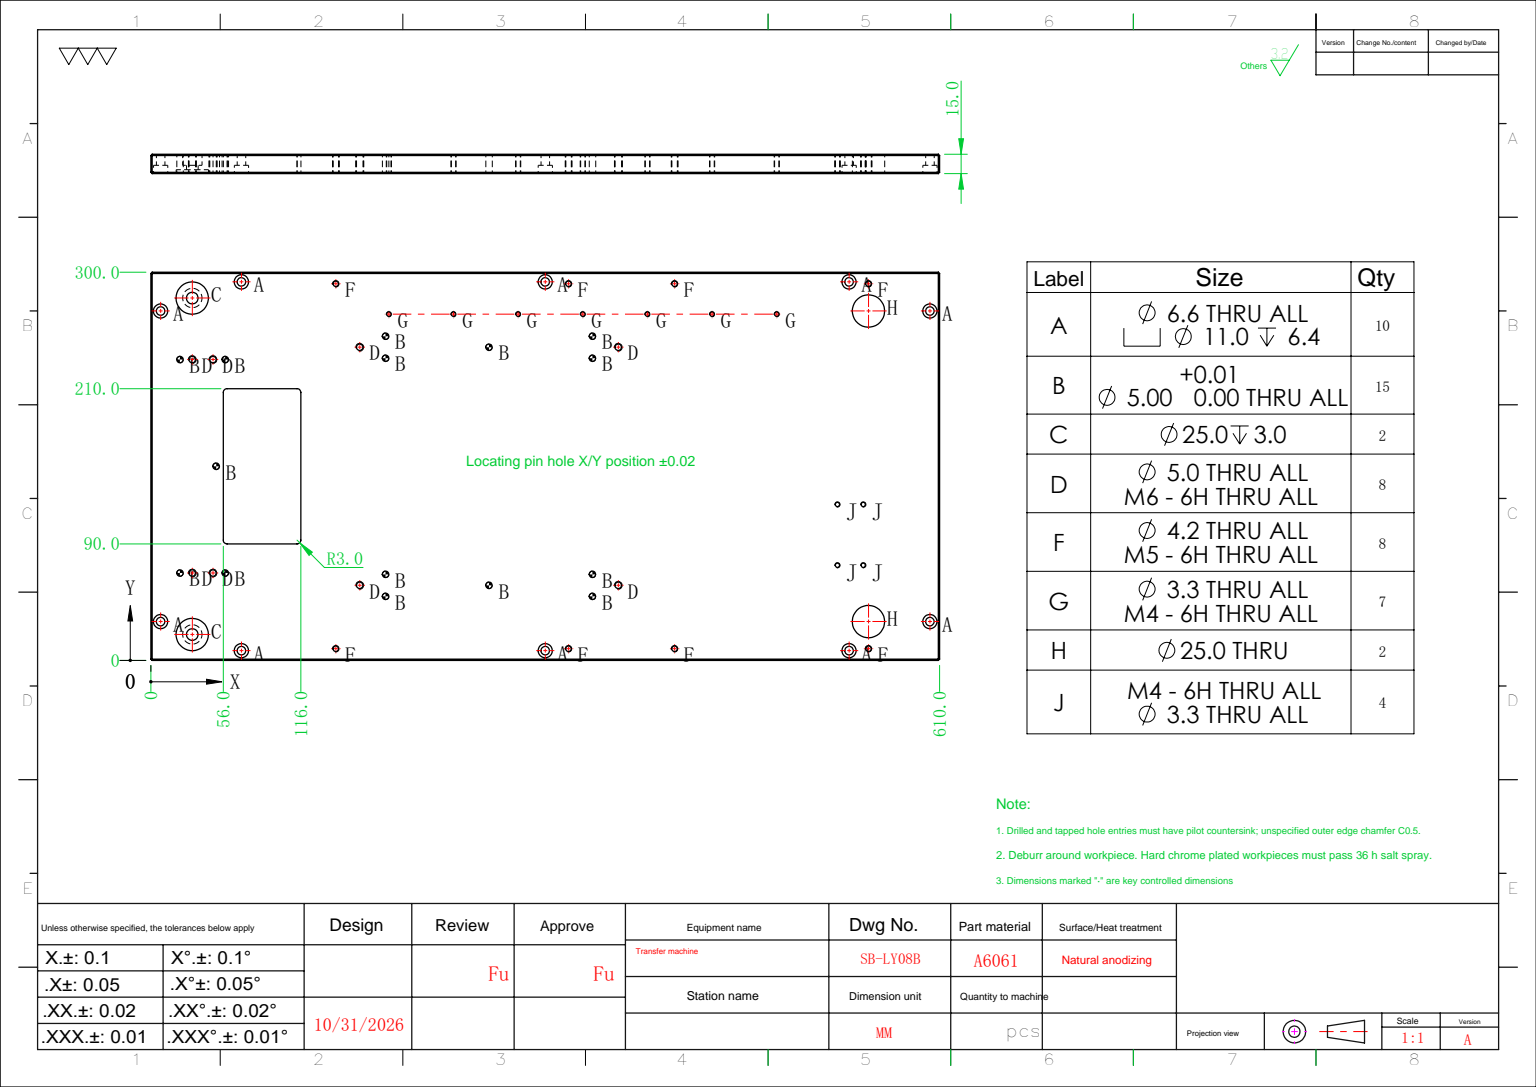
SolidWorks part; units mm, degrees
ref_plane "前视基准面" through (0, 0, 0) normal (0, 0, 1) x (1, 0, 0)
ref_plane "上视基准面" through (0, 0, 0) normal (0, 1, 0) x (1, 0, 0)
ref_plane "右视基准面" through (0, 0, 0) normal (1, 0, 0) x (0, 0, -1)
sketch "草图1" plane through (0, 0, 0) normal (0, 0, 1) x (1, 0, 0)
  line L1 (-305, -150) -> (305, -150)
  line L2 (-305, -150) -> (-305, 150)
  line L3 (-305, 150) -> (305, 150)
  line L4 (305, -150) -> (305, 150)
  line L5 (-305, -150) -> (305, 150) construction
  line L6 (-305, 150) -> (305, -150) construction
  point P0 (0, 0)
  dimension "D1" = 610
  dimension "D2" = 300
extrude "凸台-拉伸1" add sketch "草图1" along normal blind 15
sketch "草图25" plane through (0, 0, 15) normal (0, 0, 1) x (1, 0, 0)
  line L0 (0, 0) -> (254.8219, 0) construction
  line L1 (305, -150) -> (305, 150) construction
  circle A0 centre (273, -130) radius 12.5
  circle A1 centre (273, 130) radius 12.5
  dimension "D1" = 25
  dimension "D2" = 260
  dimension "D3" = 32
extrude "切除-拉伸4" cut sketch "草图25" against normal blind 3
sketch "草图26" plane through (0, 0, 15) normal (0, 0, 1) x (1, 0, 0)
  line L0 (0, 0) -> (330.7234, 0) construction
  line L1 (189, -60) -> (249, -60)
  line L2 (189, -60) -> (189, 60)
  line L3 (189, 60) -> (249, 60)
  line L4 (249, -60) -> (249, 60)
  line L5 (305, -150) -> (305, 150) construction
  dimension "D1" = 120
  dimension "D2" = 56
  dimension "D3" = 60
extrude "切除-拉伸5" cut sketch "草图26" against normal through all
hole_wizard "M6 螺纹孔1" positions "草图27" profile "草图28" tap size "M6" standard "ISO" end condition through all
sketch "草图27" plane through (0, 0, 15) normal (0, 0, 1) x (1, 0, 0)
  line L0 (0, 0) -> (315.5275, 0) construction
  line L2 (305, -150) -> (305, 150) construction
  point P0 (143.5008, -92)
  point P3 (-56.4992, -92)
  point P12 (-56.4992, 92)
  point P13 (143.5008, 92)
  dimension "D1" = 184
  dimension "D2" = 161.4992
  dimension "D3" = 200
sketch "草图28" plane through (143.5008, -92, 15) normal (1, 0, 0) x (0, -1, 0)
  line L0 (0, 0) -> (0, 15)
  line L1 (0, 15) -> (2.5, 15)
  line L2 (2.5, 15) -> (2.5, 0)
  line L5 (2.5, 0) -> (0, 0)
  line L11 (0, -6.35) -> (0, 107.95) construction
  dimension "通孔螺纹孔钻头直径" = 5
  dimension "通孔螺纹孔钻头深度" = 15
cosmetic thread "孔螺蚊线1" parameters "D2"=6
cosmetic thread "孔螺蚊线2" parameters "D2"=6
cosmetic thread "孔螺蚊线3" parameters "D2"=6
cosmetic thread "孔螺蚊线4" parameters "D2"=6
hole_wizard "大小mm 暗销孔1" positions "草图29" profile "草图30" hole size "Ø5.0" standard "ISO" end condition through all
sketch "草图29" plane through (0, 0, 15) normal (0, 0, 1) x (1, 0, 0)
  line L0 (-56.4992, -92) -> (143.5008, -92) construction
  line L3 (43.5008, -92) -> (43.5008, -134.7287) construction
  line L5 (0, 0) -> (308.2211, 0) construction
  circle A0 centre (143.5008, -92) radius 2.5 construction
  point P0 (123.5008, -83.5)
  point P2 (123.5008, -100.5)
  point P14 (43.5008, -92)
  point P18 (-36.4992, -100.5)
  point P19 (-36.4992, -83.5)
  point P25 (-36.4992, 83.5)
  point P26 (-36.4992, 100.5)
  point P27 (123.5008, 100.5)
  point P28 (123.5008, 83.5)
  point P32 (43.5008, 92)
  dimension "D1" = 17
  dimension "D2" = 20
sketch "草图30" plane through (123.5008, -83.5, 15) normal (1, 0, 0) x (0, -1, 0)
  line L0 (0, 0) -> (0, 15)
  line L1 (0, 15) -> (2.5, 15)
  line L2 (2.5, 15) -> (2.5, 0)
  line L5 (2.5, 0) -> (0, 0)
  line L11 (0, -6.35) -> (0, 107.95) construction
  dimension "通孔孔直径" = 5
  dimension "通孔孔深度" = 15
hole_wizard "M8 六角凹头螺钉的柱形沉头孔1" positions "草图31" profile "草图32" counterbore size "M8" standard "ISO" end condition through all
sketch "草图31" plane through (0, 0, 0) normal (0, 0, -1) x (-1, 0, 0)
  point P0 (-273, -130)
  point P3 (-273, 130)
sketch "草图32" plane through (273, -130, 0) normal (1, 0, 0) x (0, 1, 0)
  line L0 (0, 0) -> (0, 15)
  line L1 (0, 15) -> (4.5, 15)
  line L3 (4.5, 15) -> (4.5, 8.6)
  line L4 (4.5, 8.6) -> (7.5, 8.6)
  line L5 (7.5, 8.6) -> (7.5, 0)
  line L7 (7.5, 0) -> (0, 0)
  line L11 (0, -6.35) -> (0, 107.95) construction
  dimension "通孔孔直径" = 9
  dimension "通孔孔深度" = 15
  dimension "柱形沉头孔直径" = 15
  dimension "柱形沉头孔深度" = 8.6
hole_wizard "大小mm 暗销孔0" positions "草图33" profile "草图34" hole size "Ø5.0" standard "ISO" end condition through all
sketch "草图33" plane through (0, 0, 15) normal (0, 0, 1) x (1, 0, 0)
  line L0 (305, 0) -> (216.232, 0) construction
  line L1 (305, -150) -> (305, 150) construction
  line L2 (265, -90) -> (265, 90) construction
  point P0 (282.5, -82.5)
  point P2 (282.5, 82.5)
  point P33 (247.5, 82.5)
  point P34 (247.5, -82.5)
  point P35 (254.5, 0)
  dimension "D1" = 165
  dimension "D2" = 22.5
  dimension "D3" = 40
  dimension "D4" = 28
sketch "草图34" plane through (282.5, -82.5, 15) normal (1, 0, 0) x (0, -1, 0)
  line L0 (0, 0) -> (0, 15)
  line L1 (0, 15) -> (2.5, 15)
  line L2 (2.5, 15) -> (2.5, 0)
  line L5 (2.5, 0) -> (0, 0)
  line L11 (0, -6.35) -> (0, 107.95) construction
  dimension "通孔孔直径" = 5
  dimension "通孔孔深度" = 15
hole_wizard "M6 螺纹孔2" positions "草图35" profile "草图36" tap size "M6" standard "ISO" end condition through all
sketch "草图35" plane through (0, 0, 15) normal (0, 0, 1) x (1, 0, 0)
  line L0 (0, 0) -> (295.9256, 0) construction
  line L2 (305, -150) -> (305, 150) construction
  point P0 (257, -82.5)
  point P3 (273, -82.5)
  point P6 (257, 82.5)
  point P9 (273, 82.5)
  dimension "D1" = 165
  dimension "D2" = 32
  dimension "D3" = 16
sketch "草图36" plane through (257, -82.5, 15) normal (1, 0, 0) x (0, -1, 0)
  line L0 (0, 0) -> (0, 15)
  line L1 (0, 15) -> (2.5, 15)
  line L2 (2.5, 15) -> (2.5, 0)
  line L5 (2.5, 0) -> (0, 0)
  line L11 (0, -6.35) -> (0, 107.95) construction
  dimension "通孔螺纹孔钻头直径" = 5
  dimension "通孔螺纹孔钻头深度" = 15
cosmetic thread "孔螺蚊线5" parameters "D2"=6
cosmetic thread "孔螺蚊线6" parameters "D2"=6
cosmetic thread "孔螺蚊线7" parameters "D2"=6
cosmetic thread "孔螺蚊线8" parameters "D2"=6
hole_wizard "M6 六角凹头螺钉的柱形沉头孔1" positions "草图39" profile "草图40" counterbore size "M6" standard "ISO" end condition through all
sketch "草图39" plane through (0, 0, 15) normal (0, 0, 1) x (1, 0, 0)
  line L0 (-305, -150) -> (305, -150) construction
  line L1 (-305, 150) -> (-305, -150) construction
  line L2 (-305, 0) -> (-191.0012, 0) construction
  line L4 (0, -150) -> (0, 150) construction
  line L5 (305, 150) -> (-305, 150) construction
  point P0 (-297.5, -120)
  point P2 (-235, -142.5)
  point P13 (-235, 142.5)
  point P14 (-297.5, 120)
  point P21 (297.5, 120)
  point P22 (235, 142.5)
  point P23 (235, -142.5)
  point P24 (297.5, -120)
  point P25 (0, -142.5)
  point P28 (0, 142.5)
  dimension "D1" = 30
  dimension "D2" = 70
  dimension "D3" = 7.5
  dimension "D4" = 7.5
sketch "草图40" plane through (-297.5, -120, 15) normal (1, 0, 0) x (0, -1, 0)
  line L0 (0, 0) -> (0, 15)
  line L1 (0, 15) -> (3.3, 15)
  line L3 (3.3, 15) -> (3.3, 6.4)
  line L4 (3.3, 6.4) -> (5.5, 6.4)
  line L5 (5.5, 6.4) -> (5.5, 0)
  line L7 (5.5, 0) -> (0, 0)
  line L11 (0, -6.35) -> (0, 107.95) construction
  dimension "通孔孔直径" = 6.6
  dimension "通孔孔深度" = 15
  dimension "柱形沉头孔直径" = 11
  dimension "柱形沉头孔深度" = 6.4
hole_wizard "M4 螺纹孔1" positions "草图43" profile "草图42" tap size "M4" standard "ISO" end condition through all
sketch "草图43" plane through (0, 0, 15) normal (0, 0, 1) x (1, 0, 0)
  line L4 (-305, -150) -> (305, -150) construction
  line L5 (305, -150) -> (305, 150) construction
  point P0 (121.0008, -117.5)
  dimension "D1" = 32.5
  dimension "D2" = 183.9992
sketch "草图42" plane through (121.0008, -117.5, 15) normal (1, 0, 0) x (0, -1, 0)
  line L0 (0, 0) -> (0, 15)
  line L1 (0, 15) -> (1.65, 15)
  line L2 (1.65, 15) -> (1.65, 0)
  line L5 (1.65, 0) -> (0, 0)
  line L11 (0, -6.35) -> (0, 107.95) construction
  dimension "通孔螺纹孔钻头直径" = 3.3
  dimension "通孔螺纹孔钻头深度" = 15
cosmetic thread "孔螺蚊线9" parameters "D2"=4
pattern_linear "阵列(线性)1" count 7 spacing 50 along (-1, 0, 0) of "M4 螺纹孔1"
hole_wizard "M5 螺纹孔1" positions "草图44" profile "草图45" tap size "M5" standard "ISO" end condition through all
sketch "草图44" plane through (0, 0, 15) normal (0, 0, 1) x (1, 0, 0)
  line L8 (0, 0) -> (-330.013, 0) construction
  line L10 (-305, 150) -> (-305, -150) construction
  line L19 (-305, 150) -> (-305, -150) construction
  point P0 (-100, -141.0016)
  point P22 (-250, -141.0016)
  point P30 (-250, 141.0016)
  point P31 (-100, 141.0016)
  point P35 (-18, 141.0016)
  point P37 (162, 141.0016)
  point P58 (162, -141.0016)
  point P59 (-18, -141.0016)
  dimension "D1" = 150
  dimension "D2" = 282.0032
  dimension "D3" = 55
  dimension "D4" = 287
  dimension "D5" = 180
sketch "草图45" plane through (-100, -141.0016, 15) normal (1, 0, 0) x (0, -1, 0)
  line L0 (0, 0) -> (0, 15)
  line L1 (0, 15) -> (2.1, 15)
  line L2 (2.1, 15) -> (2.1, 0)
  line L5 (2.1, 0) -> (0, 0)
  line L11 (0, -6.35) -> (0, 107.95) construction
  dimension "通孔螺纹孔钻头直径" = 4.2
  dimension "通孔螺纹孔钻头深度" = 15
cosmetic thread "孔螺蚊线10" parameters "D2"=5
cosmetic thread "孔螺蚊线11" parameters "D2"=5
cosmetic thread "孔螺蚊线12" parameters "D2"=5
cosmetic thread "孔螺蚊线13" parameters "D2"=5
cosmetic thread "孔螺蚊线14" parameters "D2"=5
cosmetic thread "孔螺蚊线15" parameters "D2"=5
cosmetic thread "孔螺蚊线16" parameters "D2"=5
cosmetic thread "孔螺蚊线17" parameters "D2"=5
sketch "草图46" plane through (0, 0, 15) normal (0, 0, 1) x (1, 0, 0)
  line L0 (0, 0) -> (-378.3056, 0) construction
  line L1 (-305, 150) -> (-305, -150) construction
  circle A0 centre (-250, -120) radius 12.5
  circle A1 centre (-250, 120) radius 12.5
  dimension "D1" = 25
  dimension "D2" = 240
  dimension "D3" = 55
extrude "切除-拉伸6" cut sketch "草图46" against normal through all
chamfer "倒角1" distance 1 angle 45 12 edges at (0, -150, 15) (0, -150, 0) (-305, 0, 15) (-305, -150, 7.5) (-305, 0, 0) (305, -150, 7.5) (305, 0, 15) (305, 0, 0) (305, 150, 7.5) (0, 150, 15) (-305, 150, 7.5) (0, 150, 0)
hole_wizard "M4 螺纹孔2" positions "草图47" profile "草图48" tap size "M4" standard "GB" end condition through all
sketch "草图47" plane through (0, 0, 15) normal (0, 0, 1) x (1, 0, 0)
  line L0 (-305, -149) -> (-305, 149) construction
  line L1 (-304, 150) -> (304, 150) construction
  point P0 (-246, 76.5)
  point P3 (-226, 76.5)
  point P6 (-246, 29.5)
  point P9 (-226, 29.5)
  dimension "D1" = 20
  dimension "D2" = 47
  dimension "D3" = 59
  dimension "D4" = 73.5
sketch "草图48" plane through (-246, 76.5, 15) normal (1, 0, 0) x (0, -1, 0)
  line L0 (0, 0) -> (0, 15)
  line L1 (0, 15) -> (1.65, 15)
  line L2 (1.65, 15) -> (1.65, 0)
  line L5 (1.65, 0) -> (0, 0)
  line L11 (0, -6.35) -> (0, 107.95) construction
  dimension "通孔螺纹孔钻头直径" = 3.3
  dimension "通孔螺纹孔钻头深度" = 15
cosmetic thread "孔螺蚊线18" parameters "D2"=4
cosmetic thread "孔螺蚊线19" parameters "D2"=4
cosmetic thread "孔螺蚊线20" parameters "D2"=4
cosmetic thread "孔螺蚊线21" parameters "D2"=4
fillet "圆角1" radius 3 4 edges at (189, 60, 7.5) (249, 60, 7.5) (189, -60, 7.5) (249, -60, 7.5)
